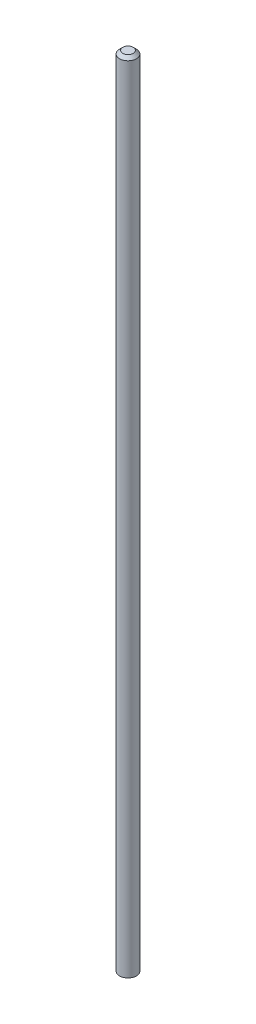
SolidWorks part; units mm, degrees
ref_plane "Front Plane" through (0, 0, 0) normal (0, 0, 1) x (1, 0, 0)
ref_plane "Top Plane" through (0, 0, 0) normal (0, 1, 0) x (1, 0, 0)
ref_plane "Right Plane" through (0, 0, 0) normal (1, 0, 0) x (0, 0, -1)
sketch "Sketch1" plane through (0, 0, 0) normal (0, 1, 0) x (1, 0, 0)
  circle A0 centre (0, 0) radius 8
  dimension "D1" = 16
extrude "Boss-Extrude1" add sketch "Sketch1" along normal blind 759
cosmetic thread "Cosmetic Thread1" parameters "D1"=30, "D2"=14
cosmetic thread "Cosmetic Thread2" parameters "D1"=30, "D2"=14
chamfer "Chamfer1" distance 3 angle 45 1 edges at (0, 759, 8)
